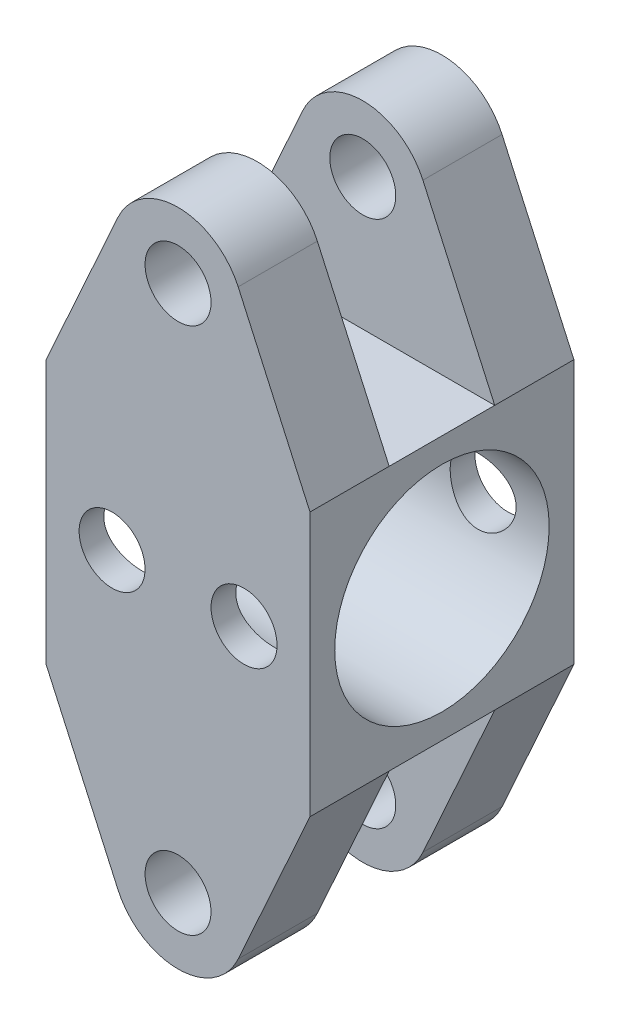
SolidWorks part; units mm, degrees
material "A3"
ref_plane "前视基准面" through (0, 0, 0) normal (0, 0, 1) x (1, 0, 0)
ref_plane "上视基准面" through (0, 0, 0) normal (0, 1, 0) x (1, 0, 0)
ref_plane "右视基准面" through (0, 0, 0) normal (1, 0, 0) x (0, 0, -1)
sketch "草图1" plane through (0, 0, 0) normal (0, 0, 1) x (1, 0, 0)
  line L0 (0, 40) -> (0, 0) construction
  line L1 (0, 0) -> (10, 0) construction
  line L2 (20, -20) -> (20, 20)
  line L3 (20, 20) -> (9.1144, 44.1144)
  line L4 (-20, -20) -> (-20, 20)
  line L5 (-20, 20) -> (-9.1144, 44.1144)
  line L6 (-20, -20) -> (-9.1144, -44.1144)
  line L7 (20, -20) -> (9.1144, -44.1144)
  circle A0 centre (0, 40) radius 5
  arc A1 (9.1144, 44.1144) -> (-9.1144, 44.1144) centre (0, 40) ccw
  circle A2 centre (10, 0) radius 5
  arc A3 (9.1144, -44.1144) -> (-9.1144, -44.1144) centre (0, -40) cw
  circle A4 centre (0, -40) radius 5
  circle A5 centre (-10, 0) radius 5
  point P18 (-20, 0)
  point P19 (20, 0)
  dimension "D1" = 10
  dimension "D2" = 20
  dimension "D3" = 40
  dimension "D4" = 10
  dimension "D5" = 40
  dimension "D6" = 40
extrude "凸台-拉伸1" add sketch "草图1" along normal mid plane 40
sketch "草图2" plane through (0, 0, 0) normal (1, 0, 0) x (0, 0, -1)
  line L0 (20, 50) -> (-20, 50) construction
  line L1 (-8, 20) -> (8, 20)
  line L2 (-8, 20) -> (-8, 80)
  line L3 (-8, 80) -> (8, 80)
  line L4 (8, 20) -> (8, 80)
  line L5 (-8, 20) -> (8, 80) construction
  line L6 (-8, 80) -> (8, 20) construction
  line L7 (-20, 20) -> (20, 20) construction
  line L8 (0, 0) -> (-20, 0) construction
  line L9 (-20, -20) -> (-20, 20) construction
  line L10 (-8, -80) -> (8, -20) construction
  line L11 (-8, -20) -> (8, -80) construction
  line L12 (8, -20) -> (8, -80)
  line L13 (-8, -80) -> (8, -80)
  line L14 (-8, -20) -> (-8, -80)
  line L15 (-8, -20) -> (8, -20)
  circle A0 centre (0, 0) radius 16.25
  point P3 (0, 50)
  point P19 (0, -50)
  dimension "D1" = 32.5
  dimension "D2" = 16
extrude "切除-拉伸1" cut sketch "草图2" against normal through all both and the other way through all
